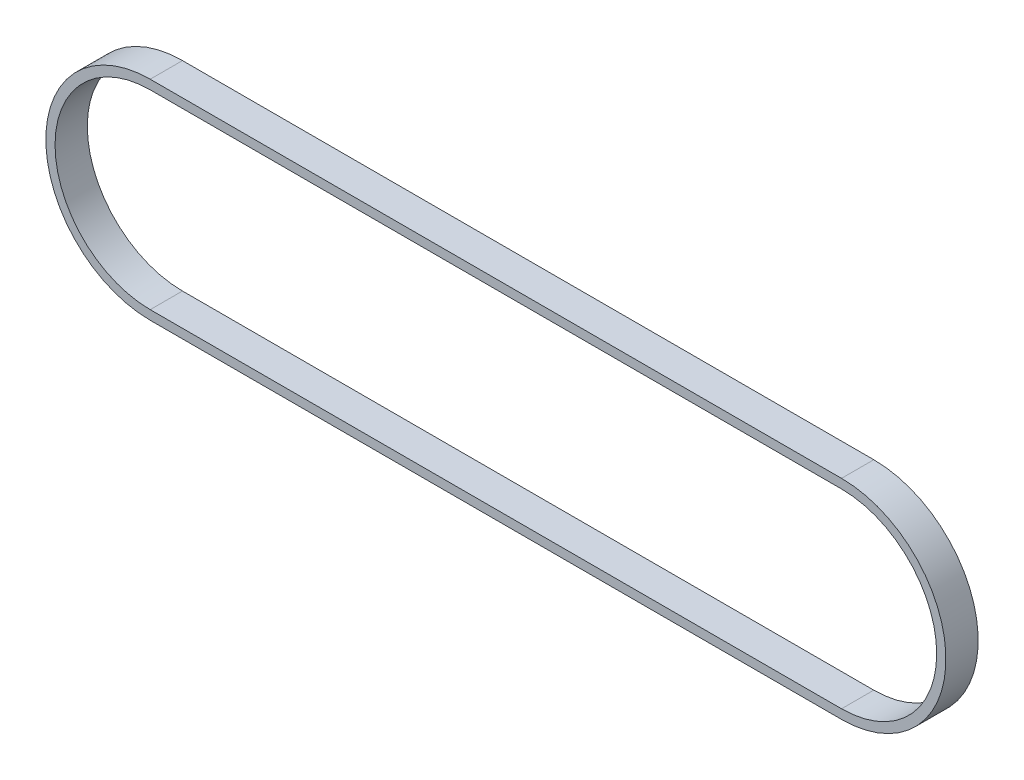
from build123d import *

# Parameters (mm, degrees)
EXTRUDE_1_DEPTH = 3.5


with BuildPart() as part:
    # 草图1 → 拉伸-薄壁1 (new, symmetric)
    with BuildSketch(Plane.XY):
        with BuildLine():
            Line((150, -22.65), (0, -22.65))
            ThreePointArc((0, -22.65), (-22.65, 0), (0, 22.65))
            Line((0, 22.65), (150, 22.65))
            ThreePointArc((150, 22.65), (172.65, 0), (150, -22.65))
        make_face()
        with BuildLine():
            Line((150, -20.65), (0, -20.65))
            ThreePointArc((0, -20.65), (-20.65, 0), (0, 20.65))
            Line((0, 20.65), (150, 20.65))
            ThreePointArc((150, 20.65), (170.65, 0), (150, -20.65))
        make_face(mode=Mode.SUBTRACT)
    extrude(amount=EXTRUDE_1_DEPTH, both=True)


solid = part.part
